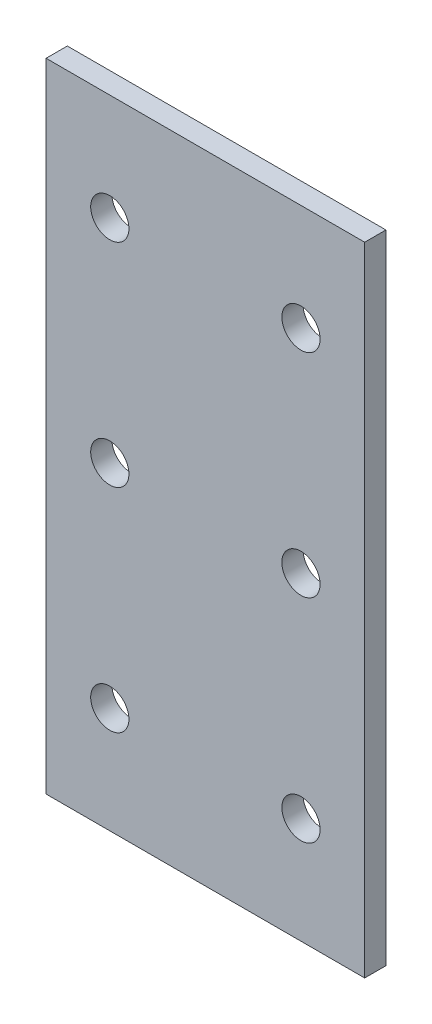
SolidWorks part; units mm, degrees
ref_plane "Front Plane" through (0, 0, 0) normal (0, 0, 1) x (1, 0, 0)
ref_plane "Top Plane" through (0, 0, 0) normal (0, 1, 0) x (1, 0, 0)
ref_plane "Right Plane" through (0, 0, 0) normal (1, 0, 0) x (0, 0, -1)
sketch "Sketch1" plane through (0, 0, 0) normal (0, 0, 1) x (1, 0, 0)
  line L0 (0, 0) -> (0, 101.2477) construction
  line L1 (75, 150) -> (-75, 150)
  line L2 (75, 150) -> (75, -150)
  line L3 (75, -150) -> (-75, -150)
  line L4 (-75, 150) -> (-75, -150)
  line L5 (75, 150) -> (-75, -150) construction
  line L6 (75, -150) -> (-75, 150) construction
  circle A0 centre (-45, 100) radius 9
  circle A2 centre (-45, 0) radius 9
  circle A3 centre (-45, -100) radius 9
  circle A4 centre (45, -100) radius 9
  circle A5 centre (45, 0) radius 9
  circle A6 centre (45, 100) radius 9
  point P0 (0, 0)
  dimension "D1" = 18
  dimension "D2" = 100
  dimension "D3" = 100
  dimension "D4" = 90
  dimension "D5" = 150
  dimension "D6" = 300
extrude "Boss-Extrude1" add sketch "Sketch1" along normal blind 10
